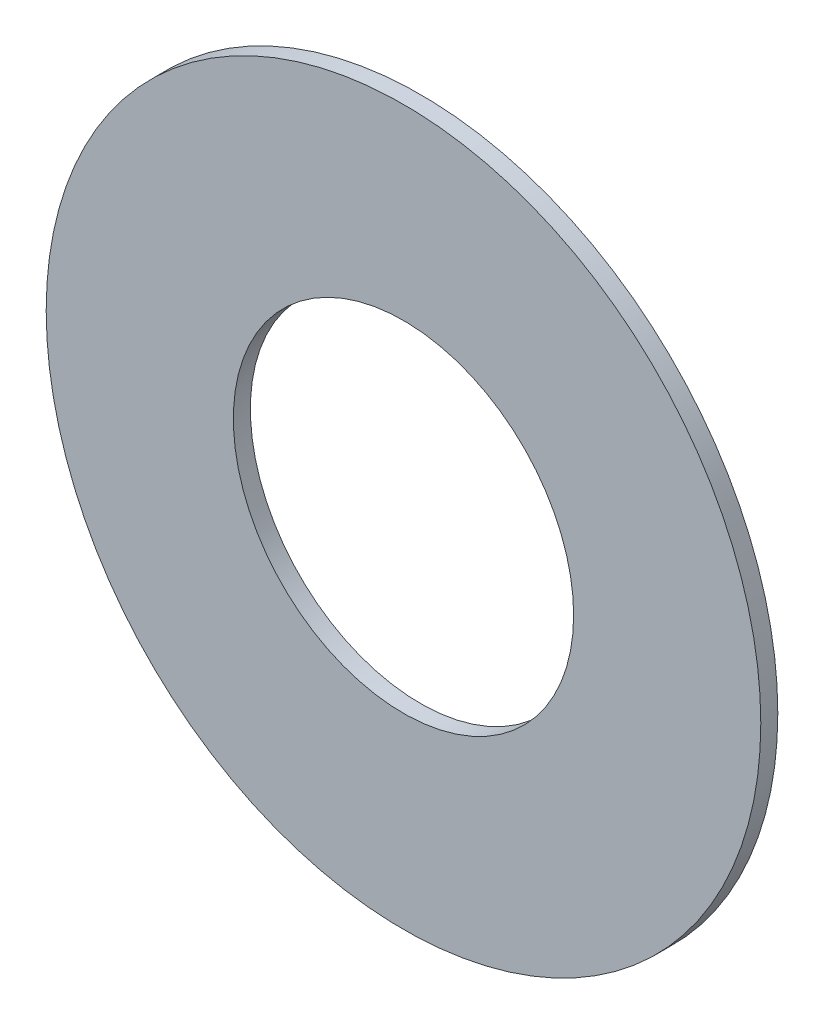
from build123d import *

# Parameters (mm, degrees)
SKETCH1_R           = 10.5
SKETCH1_R_2         = 5
BOSS_EXTRUDE1_DEPTH = 0.5


with BuildPart() as part:
    # Sketch1 → Boss-Extrude1 (new body)
    with BuildSketch(Plane.XY):
        with Locations((-121.531169153, 115.619026916)):
            Circle(SKETCH1_R)
        with Locations((-121.531169153, 115.619026916)):
            Circle(SKETCH1_R_2, mode=Mode.SUBTRACT)
    extrude(amount=BOSS_EXTRUDE1_DEPTH)


solid = part.part
